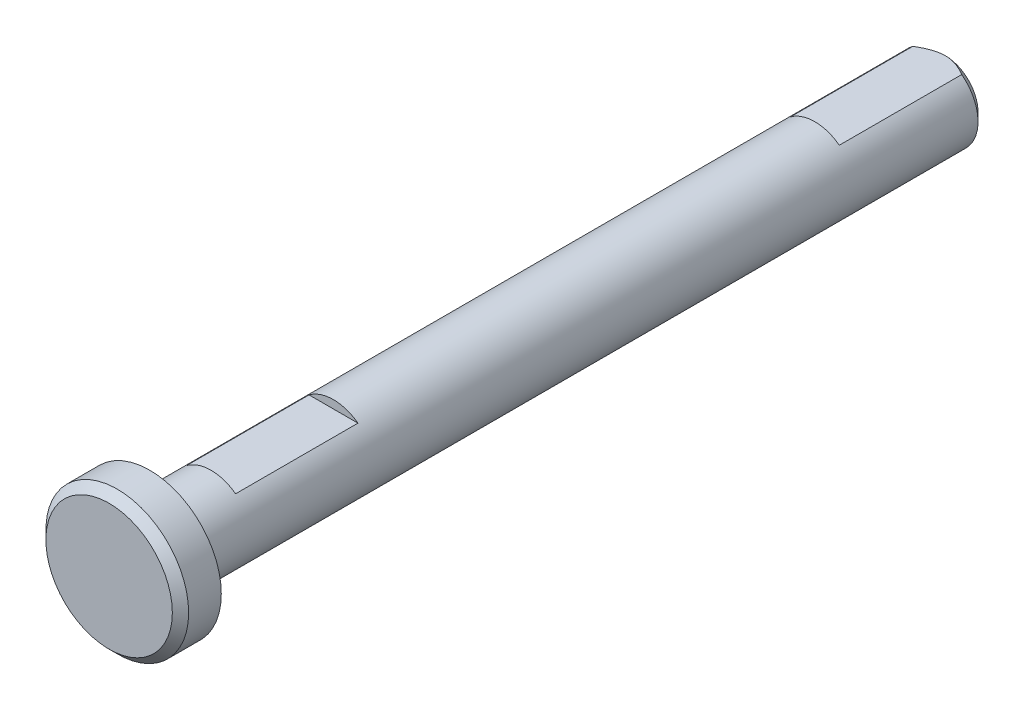
from build123d import *

# Parameters (mm, degrees)
SKETCH1_R           = 1
BOSS_EXTRUDE1_DEPTH = 9.75
SKETCH2_R           = 1.75
BOSS_EXTRUDE2_DEPTH = 1
CHAMFER1_SIZE       = 0.2
CUT_EXTRUDE1_START  = -3.2
CUT_EXTRUDE1_DEPTH  = 3.2
CUT_EXTRUDE2_DEPTH  = 1.5


with BuildPart() as part:
    # Sketch1 → Boss-Extrude1 (new, symmetric)
    with BuildSketch(Plane.XY):
        Circle(SKETCH1_R)
    extrude(amount=BOSS_EXTRUDE1_DEPTH, both=True)

    # Sketch2 → Boss-Extrude2 (add)
    with BuildSketch(Plane.XY.offset(9.75)):
        Circle(SKETCH2_R)
    extrude(amount=BOSS_EXTRUDE2_DEPTH)

    # Chamfer1
    chamfer1_edges = [part.edges().sort_by_distance(p)[0] for p in [
        (-1, 0, -9.75),
        (-1.75, 0, 10.75),
    ]]
    chamfer(chamfer1_edges, length=CHAMFER1_SIZE)

    # Sketch3 → Cut-Extrude1 (cut)
    with BuildSketch(Plane(origin=(0, 0, -9.75), x_dir=(-1, 0, 0), z_dir=(0, 0, -1)).offset(CUT_EXTRUDE1_START)):
        with BuildLine():
            Line((-0.6, 0.8), (0.6, 0.8))
            ThreePointArc((0.6, 0.8), (0, 1), (-0.6, 0.8))
        make_face()
    extrude(amount=CUT_EXTRUDE1_DEPTH, mode=Mode.SUBTRACT)

    # Sketch4 → Cut-Extrude2 (cut, symmetric)
    with BuildSketch(Plane(origin=(0, 0, 6.75), x_dir=(-1, 0, 0), z_dir=(0, 0, -1))):
        with BuildLine():
            Line((-0.6, 0.8), (0.6, 0.8))
            ThreePointArc((0.6, 0.8), (0, 1), (-0.6, 0.8))
        make_face()
    extrude(amount=CUT_EXTRUDE2_DEPTH, both=True, mode=Mode.SUBTRACT)


solid = part.part
